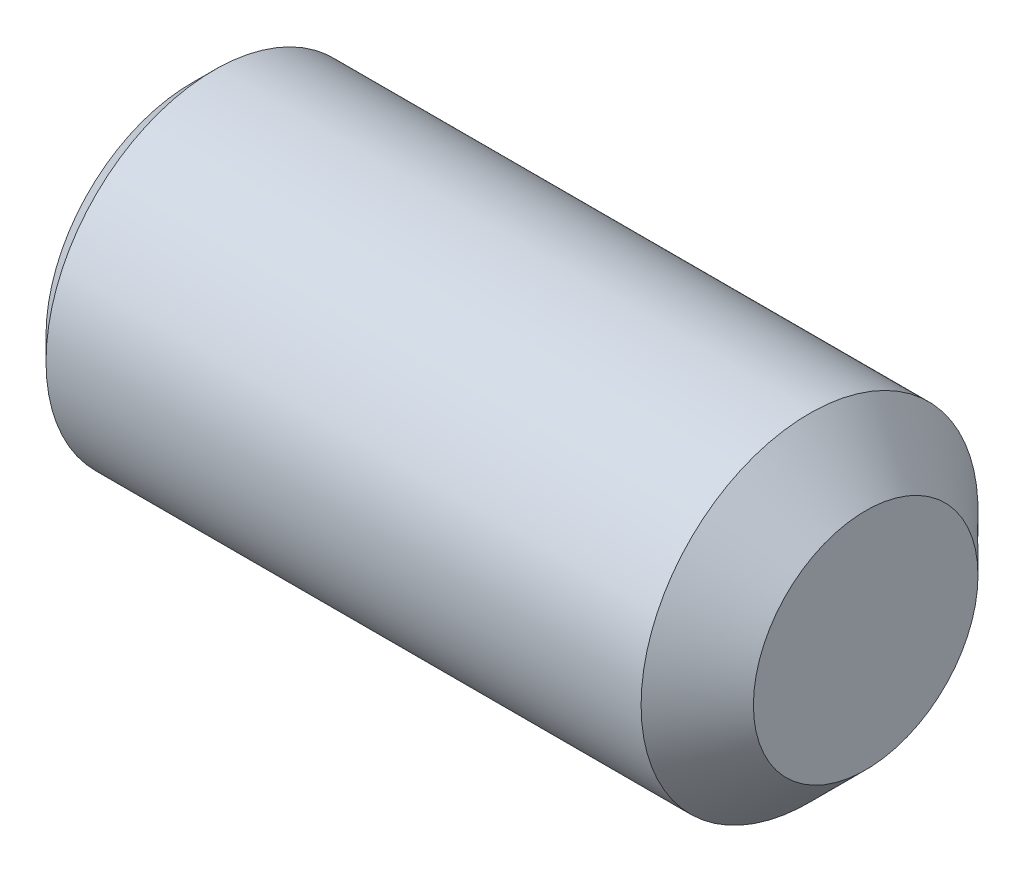
from build123d import *

# Parameters (mm, degrees)
CUT_EXTRUDE1_DEPTH = 2


with BuildPart() as part:
    # Sketch1 → Base-Revolve (revolve)
    with BuildSketch(Plane.XY, mode=Mode.PRIVATE) as base_revolve_sk:
        Polygon((0, 0), (12, 0), (12, 2), (11, 3), (0.402, 3), (0, 2.598), align=None)
    revolve(base_revolve_sk.sketch.rotate(Axis((-0.277777778, 0, 0), (1, 0, 0)), 90), axis=Axis((-0.277777778, 0, 0), (1, 0, 0)))

    # Sketch2 → Cut-Extrude1 (cut)
    with BuildSketch(Plane.ZY):
        Polygon((-0.86, -1.489563695), (0.86, -1.489563695), (1.72, 0), (0.86, 1.489563695), (-0.86, 1.489563695), (-1.72, 0), align=None)
    extrude(amount=-CUT_EXTRUDE1_DEPTH, mode=Mode.SUBTRACT)

    # Sketch4 → Cut-Revolve2 (revolve, cut)
    with BuildSketch(Plane.XY, mode=Mode.PRIVATE) as cut_revolve2_sk:
        Polygon((2, 1.489563695), (2.86, 0), (2, 0), align=None)
    revolve(cut_revolve2_sk.sketch.rotate(Axis((-0.277777778, 0, 0), (1, 0, 0)), 90), axis=Axis((-0.277777778, 0, 0), (1, 0, 0)), mode=Mode.SUBTRACT)


solid = part.part
